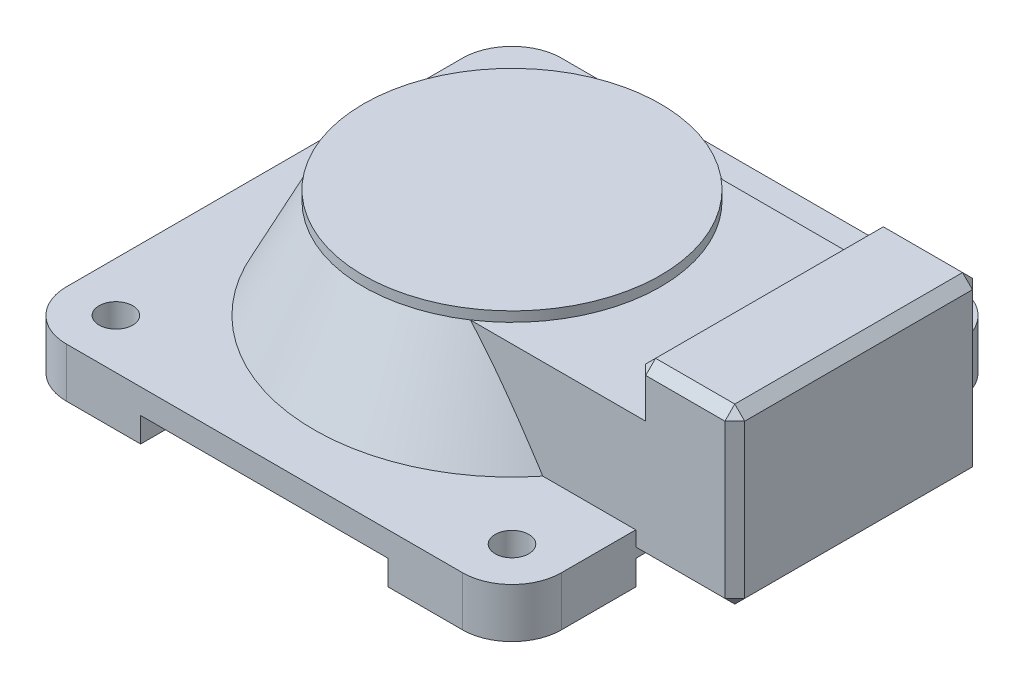
SolidWorks part; units mm, degrees
ref_plane "Front Plane" through (0, 0, 0) normal (0, 0, 1) x (1, 0, 0)
ref_plane "Top Plane" through (0, 0, 0) normal (0, 1, 0) x (1, 0, 0)
ref_plane "Right Plane" through (0, 0, 0) normal (1, 0, 0) x (0, 0, -1)
sketch "Sketch1" plane through (0, 0, 0) normal (0, 1, 0) x (1, 0, 0)
  line L1 (-50, 50) -> (50, 50)
  line L2 (-50, 50) -> (-50, -50)
  line L3 (-50, -50) -> (50, -50)
  line L4 (50, 50) -> (50, -50)
  line L5 (-50, 50) -> (50, -50) construction
  line L6 (-50, -50) -> (50, 50) construction
  point P0 (0, 0)
  dimension "D1" = 100
extrude "Boss-Extrude1" add sketch "Sketch1" along normal blind 10 contours L4 L1 L2 L3
sketch "Sketch2" plane through (0, 0, 50) normal (0, 0, 1) x (1, 0, 0)
  line L0 (-50, 0) -> (50, 0) construction
  line L1 (25, -5) -> (-25, -5)
  line L2 (25, -5) -> (25, 5)
  line L3 (25, 5) -> (-25, 5)
  line L4 (-25, -5) -> (-25, 5)
  line L5 (25, -5) -> (-25, 5) construction
  line L6 (25, 5) -> (-25, -5) construction
  point P0 (0, 0)
  dimension "D1" = 50
  dimension "D2" = 5
extrude "Cut-Extrude1" cut sketch "Sketch2" against normal through all
sketch "Sketch3" plane through (50, 0, 0) normal (1, 0, 0) x (0, 0, -1)
  line L0 (50, 0) -> (-50, 0) construction
  line L1 (25, -5) -> (-25, -5)
  line L2 (25, -5) -> (25, 5)
  line L3 (25, 5) -> (-25, 5)
  line L4 (-25, -5) -> (-25, 5)
  line L5 (25, -5) -> (-25, 5) construction
  line L6 (25, 5) -> (-25, -5) construction
  point P0 (0, 0)
  dimension "D1" = 50
  dimension "D2" = 5
extrude "Cut-Extrude2" cut sketch "Sketch3" against normal through all
fillet "Fillet1" radius 10 4 edges at (50, 5, 50) (-50, 5, 50) (-50, 5, -50) (50, 5, -50)
sketch "Sketch4" plane through (0, 0, 0) normal (0, 0, 1) x (1, 0, 0)
  line L0 (0, 10) -> (0, 30)
  line L1 (-40, 10) -> (40, 10) construction
  line L2 (0, 30) -> (30, 30)
  line L3 (30, 30) -> (40, 10)
  line L4 (40, 10) -> (0, 10)
  dimension "D1" = 20
  dimension "D2" = 30
  dimension "D3" = 40
revolve "Revolve1" add sketch "Sketch4" angle 360 about L0
sketch "Sketch5" plane through (0, 30, 0) normal (0, 1, 0) x (1, 0, 0)
  circle A1 centre (0, 0) radius 30
  circle A2 centre (0, 0) radius 30
  dimension "D1" = 0
extrude "Boss-Extrude2" add sketch "Sketch5" along normal blind 2
sketch "Sketch6" plane through (0, 0, 0) normal (1, 0, 0) x (0, 0, -1)
  line L0 (40, 10) -> (-40, 10) construction
  line L1 (-25, 30) -> (25, 30)
  line L2 (-25, 30) -> (-25, 10)
  line L3 (-25, 10) -> (25, 10)
  line L4 (25, 30) -> (25, 10)
  line L5 (-25, 30) -> (25, 10) construction
  line L6 (-25, 10) -> (25, 30) construction
  point P0 (0, 20)
  dimension "D1" = 20
  dimension "D2" = 50
extrude "Boss-Extrude3" add sketch "Sketch6" along normal up to vertex (50 mm away)
sketch "Sketch7" plane through (50, 0, 0) normal (1, 0, 0) x (0, 0, -1)
  line L0 (25, 30) -> (-25, 30) construction
  line L1 (-25, 40) -> (25, 40)
  line L2 (-25, 40) -> (-25, 5)
  line L3 (-25, 5) -> (25, 5)
  line L4 (25, 40) -> (25, 5)
  line L5 (-25, 40) -> (25, 5) construction
  line L6 (-25, 5) -> (25, 40) construction
  line L7 (25, 5) -> (-25, 5) construction
  point P0 (0, 22.5)
  dimension "D1" = 10
extrude "Boss-Extrude6" add sketch "Sketch7" along normal blind 20
chamfer "Chamfer1" distance 2 angle 45 11 edges at (70, 5, 0) (50, 40, 0) (60, 5, -25) (50, 35, -25) (60, 40, -25) (70, 22.5, -25) (70, 40, 0) (60, 5, 25) (70, 22.5, 25) (60, 40, 25) (50, 35, 25)
hole_wizard "M8 Tapped Hole1" positions "Sketch10" profile "Sketch9" tap size "M8" standard "GB"
sketch "Sketch10" plane through (0, 10, 0) normal (0, 1, 0) x (1, 0, 0)
  point P0 (40, 40)
  point P3 (40, -40)
  point P6 (-40, -40)
  point P9 (-40, 40)
sketch "Sketch9" plane through (40, 10, -40) normal (1, 0, 0) x (0, 0, 1)
  line L0 (0, 0) -> (0, 22.25)
  line L1 (0, 22.25) -> (3.4, 20.2071)
  line L2 (3.4, 20.2071) -> (3.4, 0)
  line L5 (3.4, 0) -> (0, 0)
  line L10 (0, 22.25) -> (-3.4, 20.2071) construction
  line L11 (0, -6.35) -> (0, 107.95) construction
  dimension "螺纹孔钻头直径" = 6.8
  dimension "螺纹孔钻头深度" = 22.25
  dimension "导头角度" = 118
